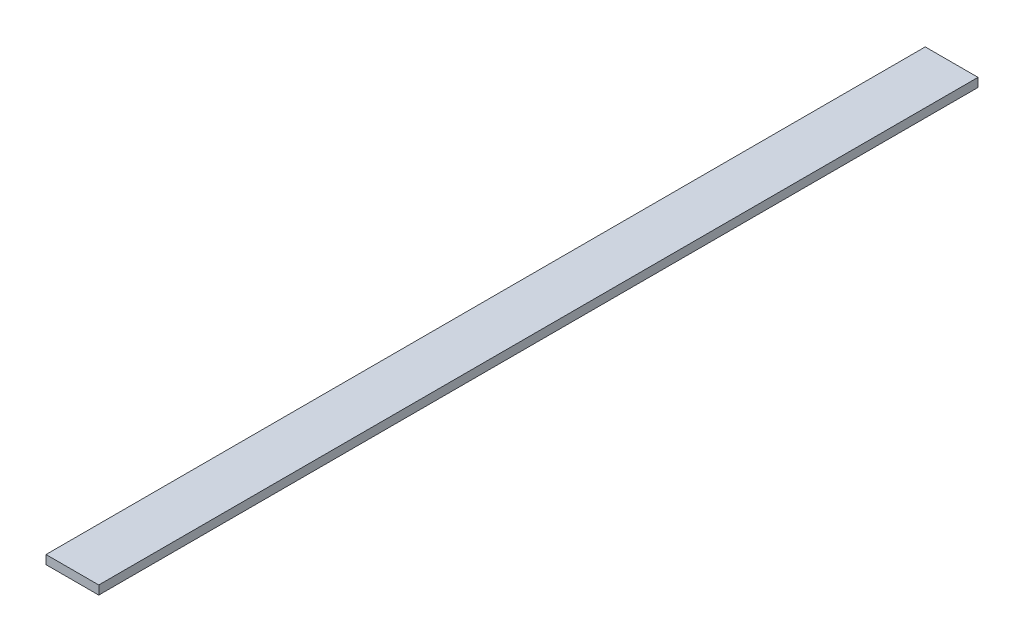
SolidWorks part; units mm, degrees
ref_plane "前视基准面" through (0, 0, 0) normal (0, 0, 1) x (1, 0, 0)
ref_plane "上视基准面" through (0, 0, 0) normal (0, 1, 0) x (1, 0, 0)
ref_plane "右视基准面" through (0, 0, 0) normal (1, 0, 0) x (0, 0, -1)
sketch "草图1" plane through (0, 0, 0) normal (0, 0, 1) x (1, 0, 0)
  line L1 (-9, 1.5) -> (9, 1.5)
  line L2 (-9, 1.5) -> (-9, -1.5)
  line L3 (-9, -1.5) -> (9, -1.5)
  line L4 (9, 1.5) -> (9, -1.5)
  line L5 (-9, 1.5) -> (9, -1.5) construction
  line L6 (-9, -1.5) -> (9, 1.5) construction
  point P0 (0, 0)
  dimension "D1" = 3
  dimension "D2" = 18
extrude "凸台-拉伸1" add sketch "草图1" along normal blind 300
